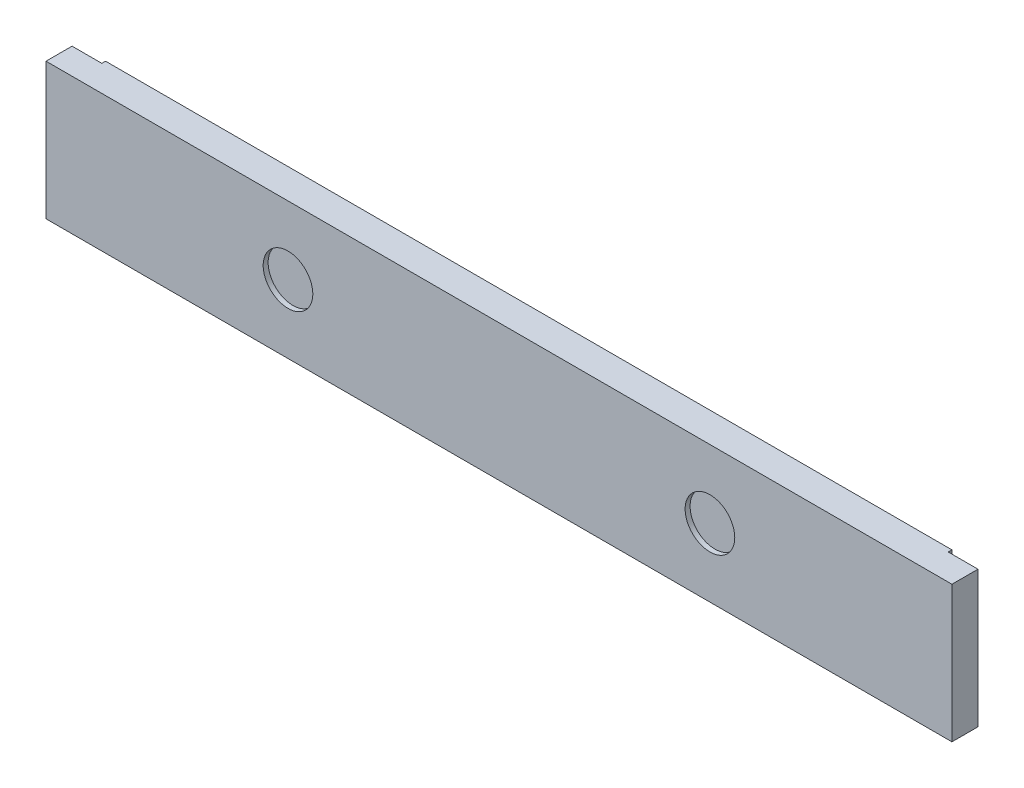
SolidWorks part; units mm, degrees
ref_plane "前视基准面" through (0, 0, 0) normal (0, 0, 1) x (1, 0, 0)
ref_plane "上视基准面" through (0, 0, 0) normal (0, 1, 0) x (1, 0, 0)
ref_plane "右视基准面" through (0, 0, 0) normal (1, 0, 0) x (0, 0, -1)
sketch "草图1" plane through (0, 0, 0) normal (0, 0, 1) x (1, 0, 0)
  line L1 (-182.5, -27.5) -> (182.5, -27.5)
  line L2 (-182.5, -27.5) -> (-182.5, 27.5)
  line L3 (-182.5, 27.5) -> (182.5, 27.5)
  line L4 (182.5, -27.5) -> (182.5, 27.5)
  line L5 (-182.5, -27.5) -> (182.5, 27.5) construction
  line L6 (-182.5, 27.5) -> (182.5, -27.5) construction
  point P0 (0, 0)
  dimension "D1" = 55
  dimension "D2" = 365
extrude "凸台-拉伸1" add sketch "草图1" along normal blind 12
sketch "草图2" plane through (0, 0, 12) normal (0, 0, 1) x (1, 0, 0)
  circle A0 centre (0, 0) radius 10.5 construction
  circle A1 centre (85, 0) radius 10
  circle A2 centre (-85, 0) radius 10
extrude "切除-拉伸1" cut sketch "草图2" against normal blind 2
sketch "草图3" plane through (0, 0, 0) normal (0, 0, -1) x (-1, 0, 0)
  line L0 (-182.5, 27.5) -> (182.5, 27.5) construction
  line L1 (182.5, -27.5) -> (170.5, -27.5)
  line L2 (182.5, -27.5) -> (182.5, 27.5)
  line L3 (182.5, 27.5) -> (170.5, 27.5)
  line L4 (170.5, -27.5) -> (170.5, 27.5)
  line L6 (-182.5, -27.5) -> (-170.5, -27.5)
  line L7 (-182.5, -27.5) -> (-182.5, 27.5)
  line L8 (-182.5, 27.5) -> (-170.5, 27.5)
  line L9 (-170.5, -27.5) -> (-170.5, 27.5)
  dimension "D1" = 12
extrude "切除-拉伸2" cut sketch "草图3" against normal blind 1.5
equation "\"D5@草图2\"=\"D4@草图2\""
